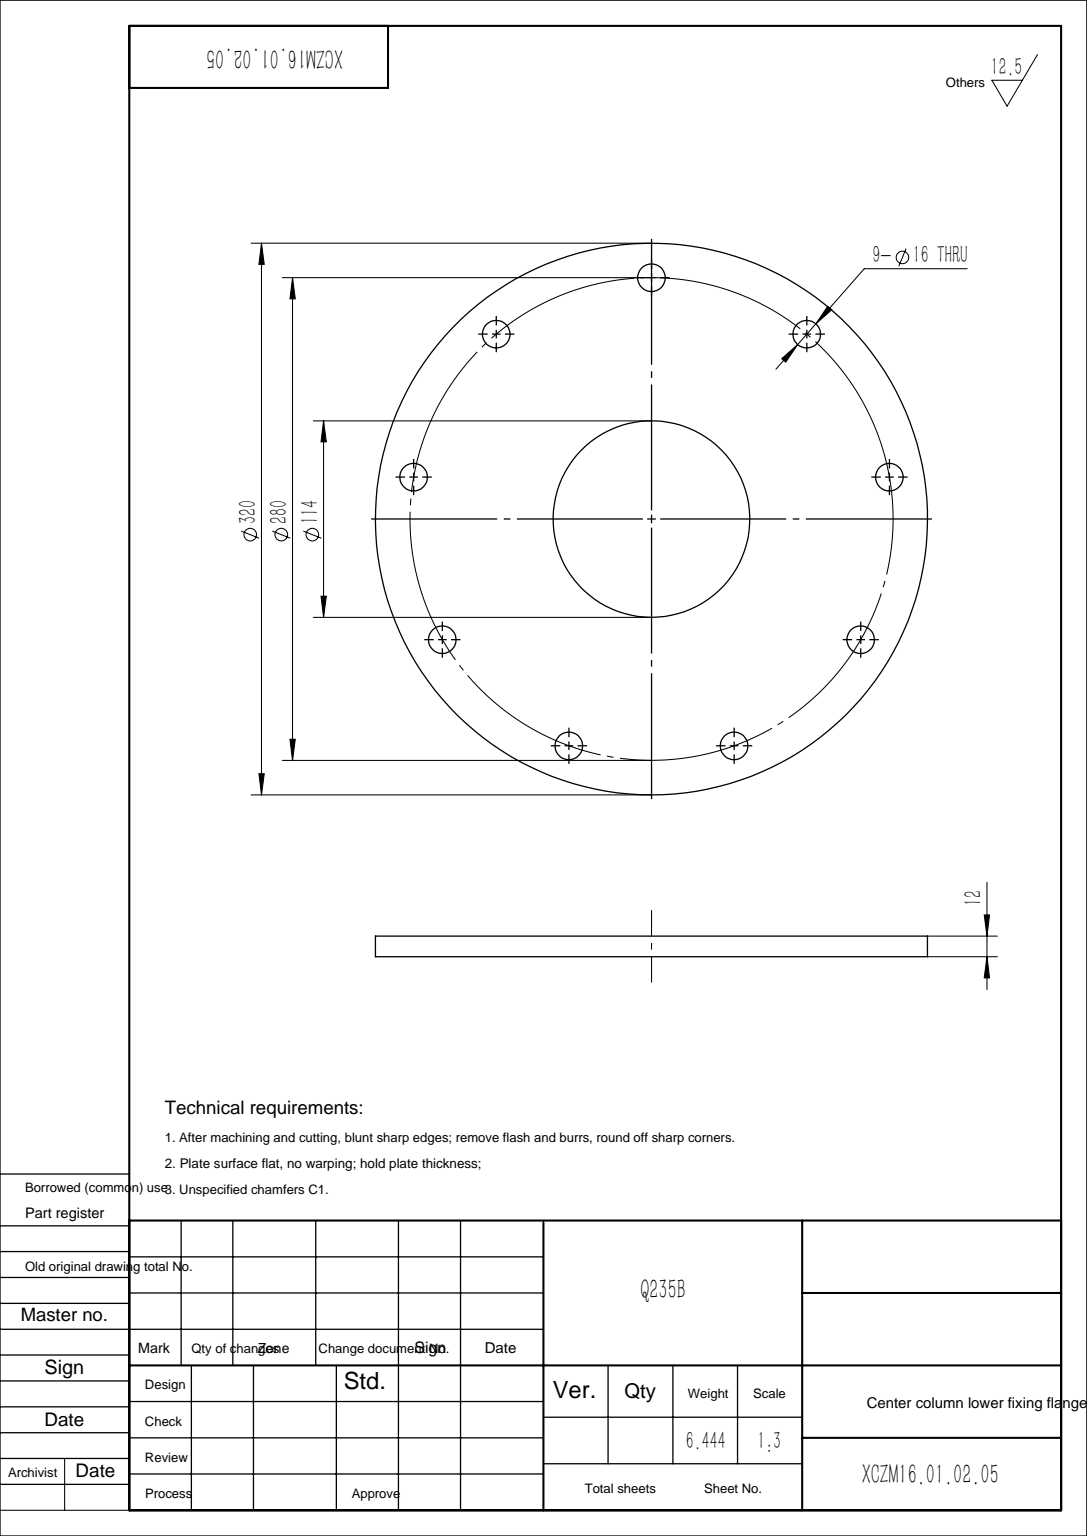
SolidWorks part; units mm, degrees
material "Q235B"
ref_plane "Front Plane" through (0, 0, 0) normal (0, 0, 1) x (1, 0, 0)
ref_plane "Top Plane" through (0, 0, 0) normal (0, 1, 0) x (1, 0, 0)
ref_plane "Right Plane" through (0, 0, 0) normal (1, 0, 0) x (0, 0, -1)
sketch "Sketch1" plane through (0, 0, 0) normal (0, 1, 0) x (1, 0, 0)
  line L0 (0, 0) -> (0, 140) construction
  line L1 (0, 0) -> (89.9903, 107.2462) construction
  circle A0 centre (0, 0) radius 57
  circle A1 centre (0, 0) radius 160
  circle A3 centre (0, 0) radius 140 construction
  circle A5 centre (0, 140) radius 8
  circle A6 centre (89.9903, 107.2462) radius 8
  circle A7 centre (137.8731, 24.3107) radius 8
  circle A8 centre (121.2436, -70) radius 8
  circle A9 centre (47.8828, -131.557) radius 8
  circle A10 centre (-47.8828, -131.557) radius 8
  circle A11 centre (-121.2436, -70) radius 8
  circle A12 centre (-137.8731, 24.3107) radius 8
  circle A13 centre (-89.9903, 107.2462) radius 8
  dimension "D1" = 114
  dimension "D2" = 320
  dimension "D4" = 280
  dimension "D6" = 16
  dimension "D8" = 40
  dimension "D7" = 9
extrude "Boss-Extrude1" add sketch "Sketch1" along normal blind 12
